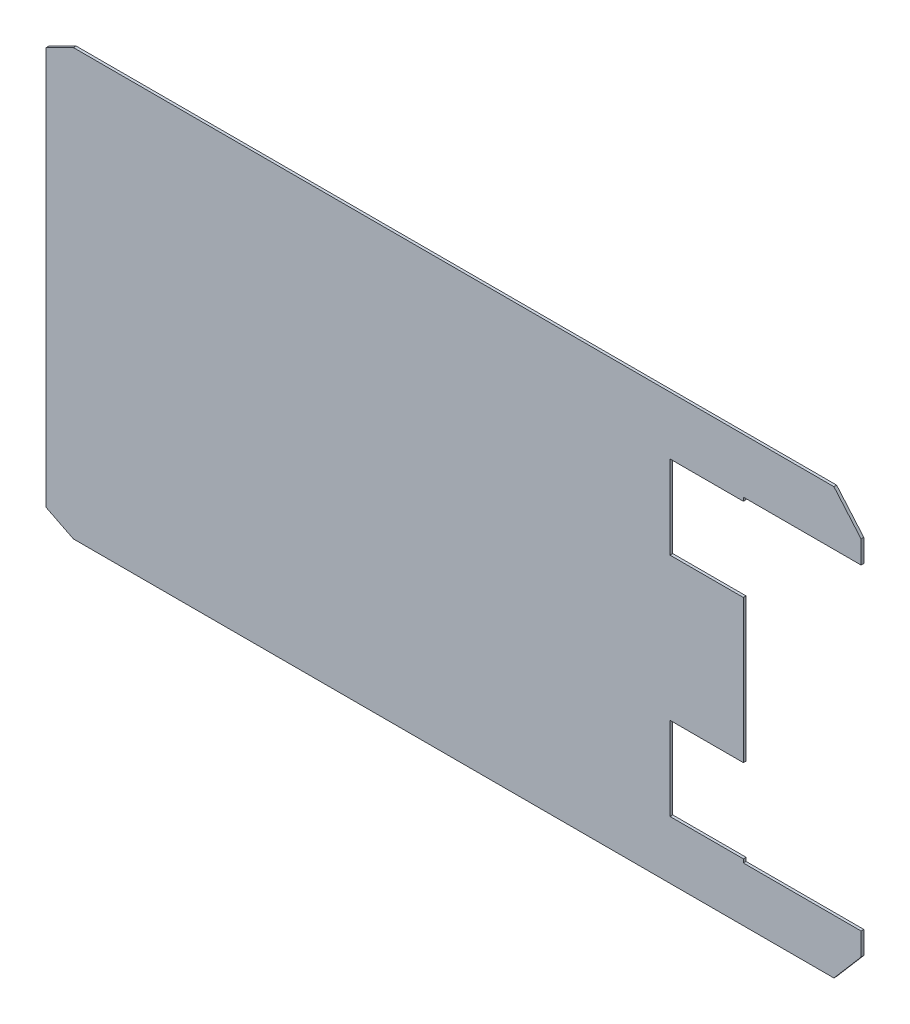
from build123d import *

# Parameters (mm, degrees)
EXTRUDE_1_DEPTH     = 1.5
SKETCH_2_W          = 102
SKETCH_2_H          = 92
CUT_EXTRUDE_1_DEPTH = 15


with BuildPart() as part:
    # 草图1 → 凸台-拉伸1 (new, symmetric)
    with BuildSketch(Plane.XY):
        Polygon((-620, -220), (-590, -235), (250, -235), (280, -200), (280, -175), (150, -175), (150, 175), (280, 175), (280, 200), (250, 235), (-590, 235), (-620, 220), align=None)
    extrude(amount=EXTRUDE_1_DEPTH, both=True)

    # 草图2 → 切除-拉伸1 (cut, symmetric)
    with BuildSketch(Plane.XY):
        with Locations((120, 125)):
            Rectangle(SKETCH_2_W, SKETCH_2_H)
        with Locations((120, -125)):
            Rectangle(SKETCH_2_W, SKETCH_2_H)
    extrude(amount=CUT_EXTRUDE_1_DEPTH, both=True, mode=Mode.SUBTRACT)


solid = part.part
